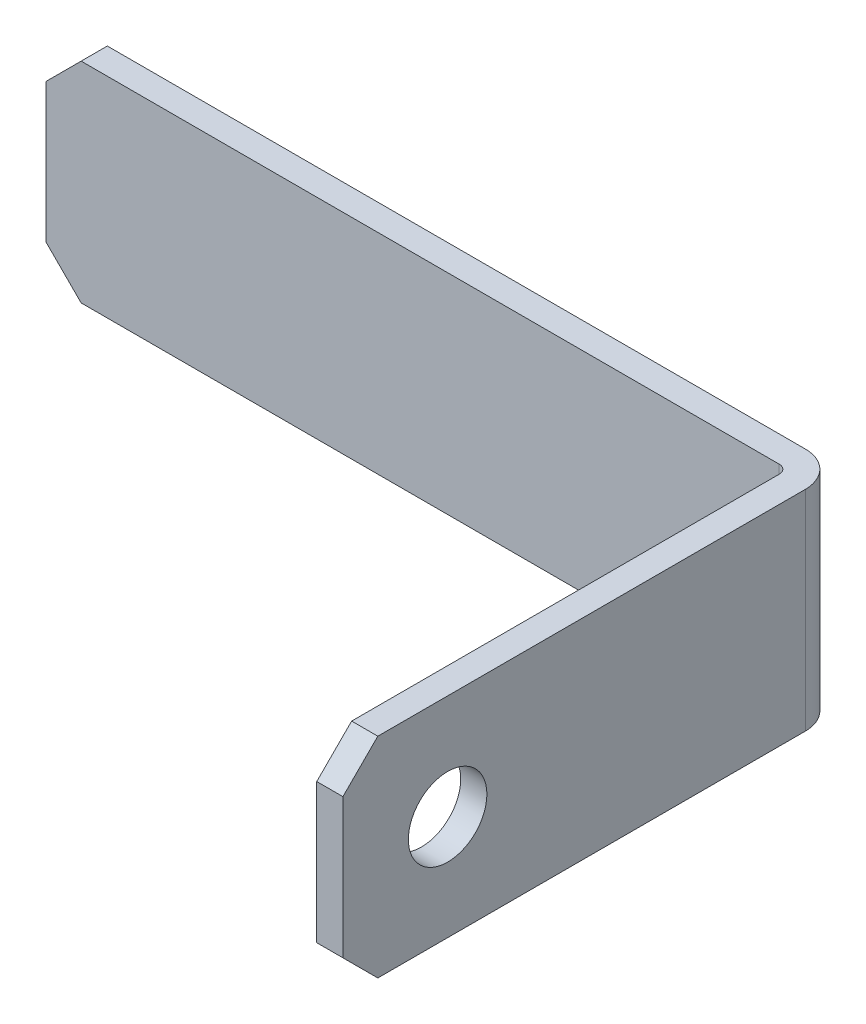
SolidWorks part; units mm, degrees
ref_plane "Front Plane" through (0, 0, 0) normal (0, 0, 1) x (1, 0, 0)
ref_plane "Top Plane" through (0, 0, 0) normal (0, 1, 0) x (1, 0, 0)
ref_plane "Right Plane" through (0, 0, 0) normal (1, 0, 0) x (0, 0, -1)
sketch "Sketch1" plane through (0, 0, 0) normal (0, 1, 0) x (1, 0, 0)
  line L1 (0, 0) -> (-1.5, 0)
  line L2 (0, 0) -> (0, 28.5)
  line L3 (0, 28.5) -> (-44, 28.5)
  line L4 (-44, 27) -> (-44, 28.5)
  line L7 (-44, 27) -> (-1.5, 27)
  line L8 (-1.5, 0) -> (-1.5, 27)
  dimension "D1" = 28.5
  dimension "D2" = 44
  dimension "D3" = 1.5
  dimension "D4" = 1.5
extrude "Boss-Extrude1" add sketch "Sketch1" along normal blind 12
sketch "Sketch2" plane through (0, 0, 0) normal (1, 0, 0) x (0, 0, -1)
  line L0 (0, 6) -> (23.8639, 6) construction
  line L1 (0, 12) -> (0, 0) construction
  circle A0 centre (6, 6) radius 2.25
  dimension "D1" = 4.5
  dimension "D2" = 6
extrude "Cut-Extrude1" cut sketch "Sketch2" against normal through all
chamfer "Chamfer1" distance 2 angle 45 4 edges at (-0.75, 0, 0) (-0.75, 12, 0) (-44, 0, -27.75) (-44, 12, -27.75)
fillet "Fillet1" radius 2 1 edges at (0, 6, -28.5)
fillet "Fillet2" radius 0.5 1 edges at (-1.5, 6, -27)
